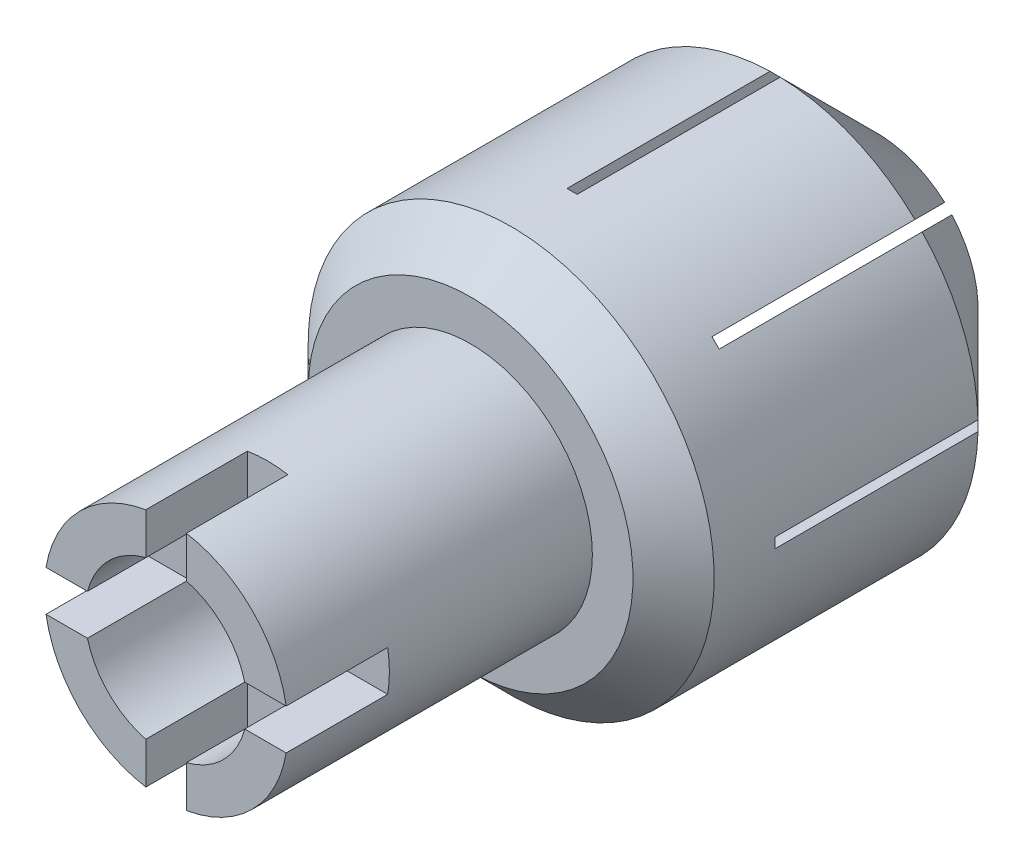
SolidWorks part; units mm, degrees
material "Brass"
ref_plane "Front Plane" through (0, 0, 0) normal (0, 0, 1) x (1, 0, 0)
ref_plane "Top Plane" through (0, 0, 0) normal (0, 1, 0) x (1, 0, 0)
ref_plane "Right Plane" through (0, 0, 0) normal (1, 0, 0) x (0, 0, -1)
other "Configuration Table"
sketch "Sketch1" plane through (0, 0, 0) normal (0, 1, 0) x (1, 0, 0)
  line L0 (0, 0) -> (10, 0)
  line L1 (10, 0) -> (10, 15)
  line L2 (10, 15) -> (5, 20)
  line L3 (5, 20) -> (0, 20)
  line L4 (0, 20) -> (0, -15) construction
  line L5 (3, 20) -> (3, 0)
  line L6 (6, 0) -> (6, -15)
  line L7 (6, -15) -> (0, -15)
  line L8 (4, 0) -> (4, -15)
  dimension "D1" = 3
  dimension "D2" = 10
  dimension "D3" = 5
  dimension "D4" = 20
  dimension "D5" = 35
  dimension "D6" = 6
  dimension "D7" = 15
  dimension "D8" = 4
  dimension "D9" = 135
  dimension "D10" = 135
revolve "Revolve1" add sketch "Sketch1" angle 360 about L4
sketch "Sketch2" plane through (0, 0, -20) normal (0, 0, -1) x (-1, 0, 0)
  line L0 (-10, 0) -> (10, 0) construction
  line L1 (0, 10) -> (0, -10) construction
  line L2 (-10, -0.25) -> (10, -0.25)
  line L3 (-0.25, 10) -> (-0.25, -10)
  line L4 (-10, 0.25) -> (10, 0.25)
  line L5 (0.25, 10) -> (0.25, -10)
  line L6 (7.0711, 7.0711) -> (-7.0711, -7.0711) construction
  line L7 (6.8943, 7.2478) -> (-7.2478, -6.8943)
  line L8 (7.2478, 6.8943) -> (-6.8943, -7.2478)
  line L9 (-7.0711, 7.0711) -> (7.0711, -7.0711) construction
  line L10 (-7.2478, 6.8943) -> (6.8943, -7.2478)
  line L11 (-6.8943, 7.2478) -> (7.2478, -6.8943)
  circle A0 centre (0, 0) radius 10 construction
  circle A2 centre (0, 0) radius 10
  circle A3 centre (0, 0) radius 10
  circle M3 centre (0, 0) radius 3
  circle M4 centre (0, 0) radius 5
  dimension "D1" = 0.25
  dimension "D4" = 45
  dimension "D5" = 0.25
  dimension "D2" = 0.25
  dimension "D3" = 0
  dimension "D6" = 0.25
extrude "Cut-Extrude1" cut sketch "Sketch2" against normal blind 15 contours L4 A3 L2 L3 | L2 A3 L4 L5 | L5 A3 L3 L4 | L3 A3 L5 L2 | L7 A3 L8 M4 | L10 A3 L11 M4 | L8 A3 L7 M4 | L11 A3 L10 M4 | L11 L10 M4 M3 | L5 L3 M4 M3 | L8 L7 M4 M3 | L4 L2 M3 M4 | L11 L10 M3 M4 | L5 L3 M3 M4 | L8 L7 M3 M4 | L4 L2 M4 M3
chamfer "Chamfer1" distance 2 angle 45 1 edges at (-10, 0, 0)
sketch "Sketch3" plane through (0, 0, 15) normal (0, 0, 1) x (1, 0, 0)
  line L0 (6, 0) -> (4, 0) construction
  line L1 (5.9161, 1) -> (3.873, 1)
  line L2 (5.9161, -1) -> (3.873, -1)
  line L3 (1000, 1) -> (-13.9682, 1) construction
  line L4 (1000, 0) -> (-13.9682, 0) construction
  line L5 (1000, -1) -> (-13.9682, -1) construction
  line L6 (0, 6) -> (0, 4) construction
  line L7 (-1, 6) -> (-1, 3.873)
  line L8 (1, 6) -> (1, 3.873)
  line L10 (1, 6) -> (1, -6) construction
  line L12 (0, 6) -> (0, -6) construction
  line L14 (-1, 6) -> (-1, -6) construction
  line L15 (-3.873, 1) -> (-5.9161, 1)
  line L16 (-4, 0) -> (-6, 0) construction
  line L17 (-3.873, -1) -> (-5.9161, -1)
  line L18 (-1, -3.873) -> (-1, -6)
  line L19 (0, -4) -> (0, -6) construction
  line L20 (1, -3.873) -> (1, -6)
  circle A0 centre (0, 0) radius 4 construction
  circle A1 centre (0, 0) radius 4
  circle A5 centre (0, 0) radius 6
  circle A6 centre (0, 0) radius 6
  circle M6 centre (0, 0) radius 4
  circle M7 centre (0, 0) radius 6
  dimension "D6" = 12
  dimension "D1" = 1
  dimension "D2" = 1
  dimension "D3" = 1
  dimension "D4" = 1
  dimension "D5" = 0
extrude "Cut-Extrude2" cut sketch "Sketch3" against normal blind 5 contours L8 L7 M7 M6 | L2 L1 M7 M6 | L20 L18 M6 M7 | L17 L15 M6 M7
